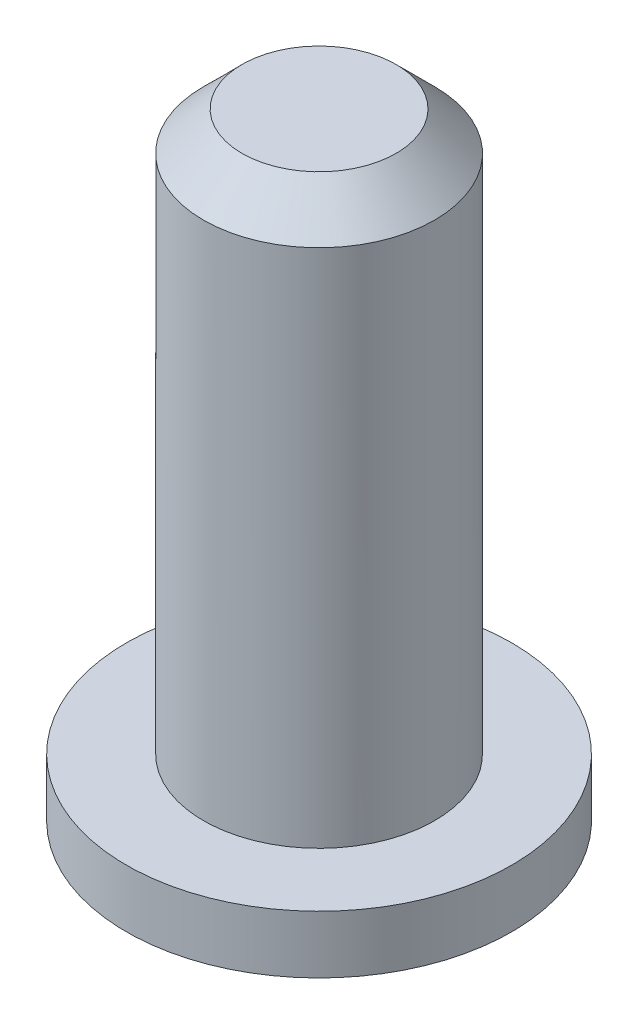
from build123d import *

# Parameters (mm, degrees)
CHAMFER1_SIZE = 2


with BuildPart() as part:
    # Sketch1 → Revolve1 (revolve)
    with BuildSketch(Plane.XY, mode=Mode.PRIVATE) as revolve1_sk:
        Polygon((0, 0), (10, 0), (10, 3), (6, 3), (6, 32), (0, 32), align=None)
    revolve(revolve1_sk.sketch.rotate(Axis((0, 0, 0), (0, 1, 0)), 90), axis=Axis((0, 0, 0), (0, 1, 0)))

    # Chamfer1
    chamfer1_edges = [part.edges().sort_by_distance(p)[0] for p in [
        (0, 32, 6),
    ]]
    chamfer(chamfer1_edges, length=CHAMFER1_SIZE)


solid = part.part
